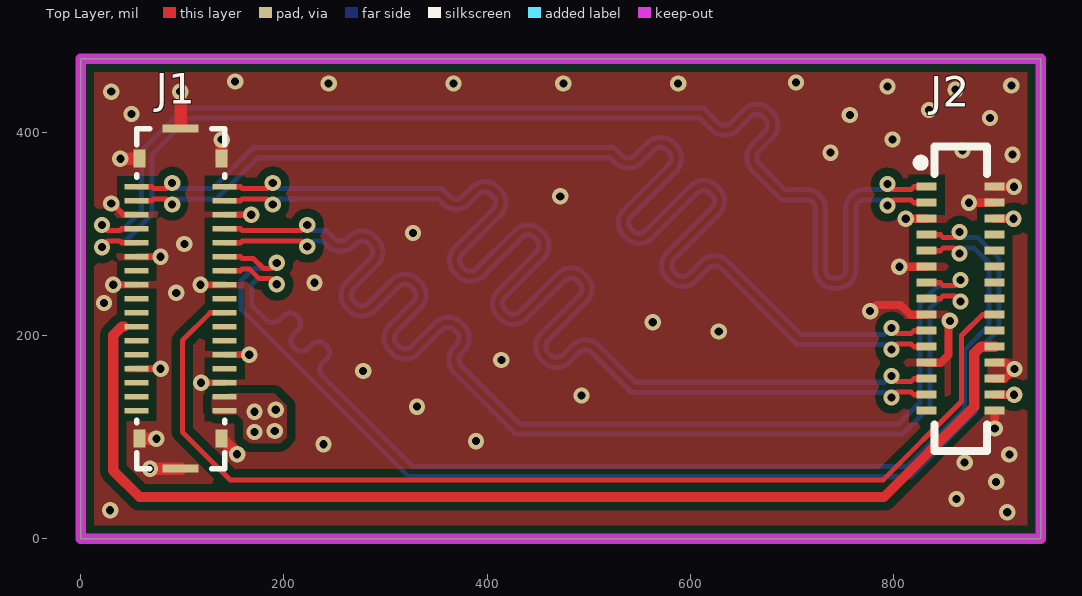
[diagram p0: Top Layer view]
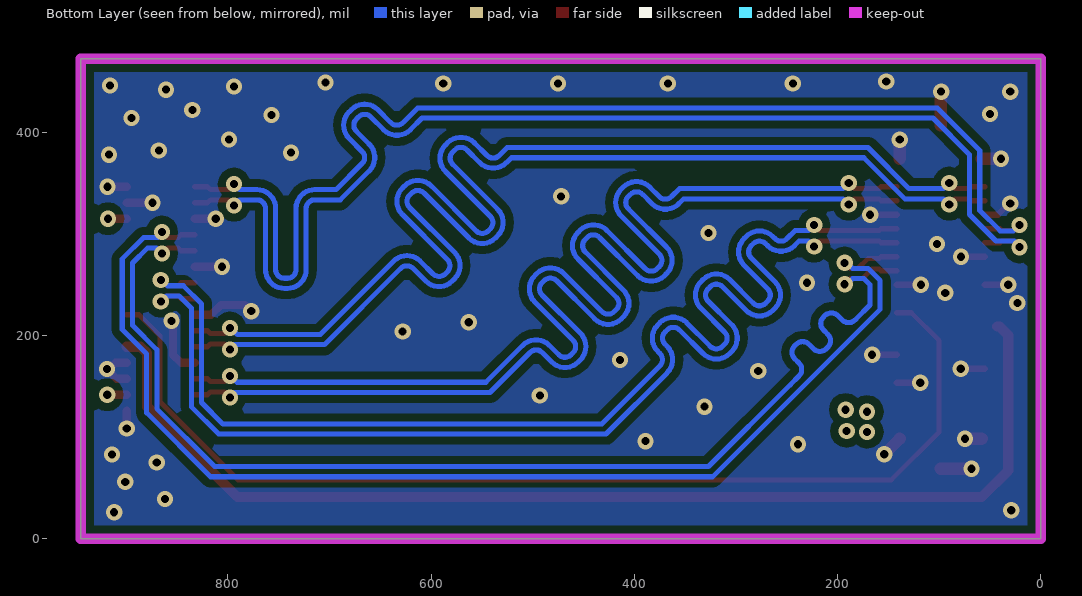
[diagram p1: Bottom Layer view, seen from below]
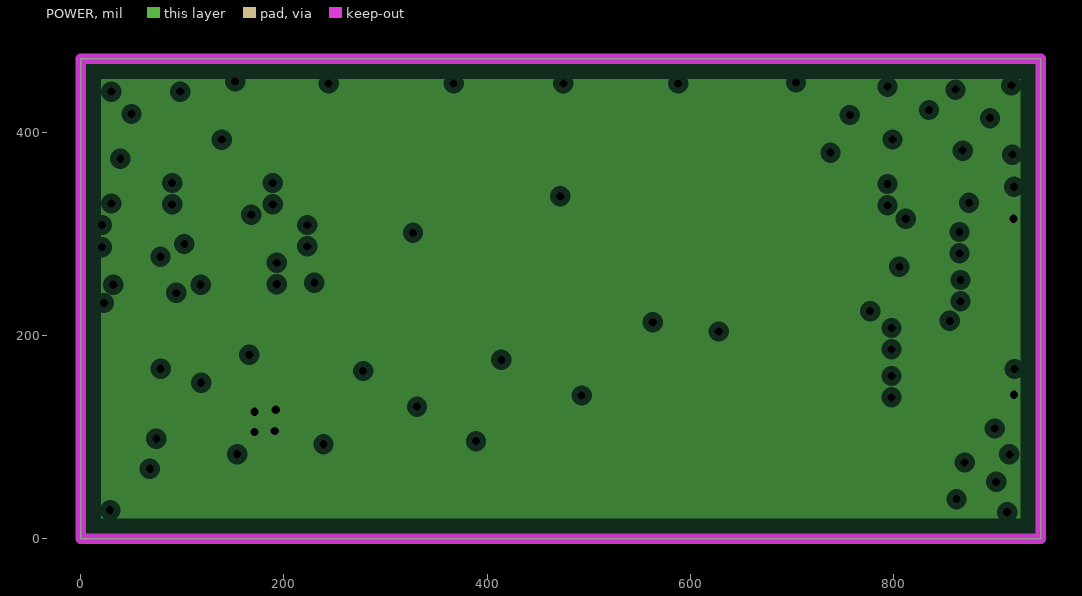
[diagram p2: POWER, clearances drawn from the general rule]
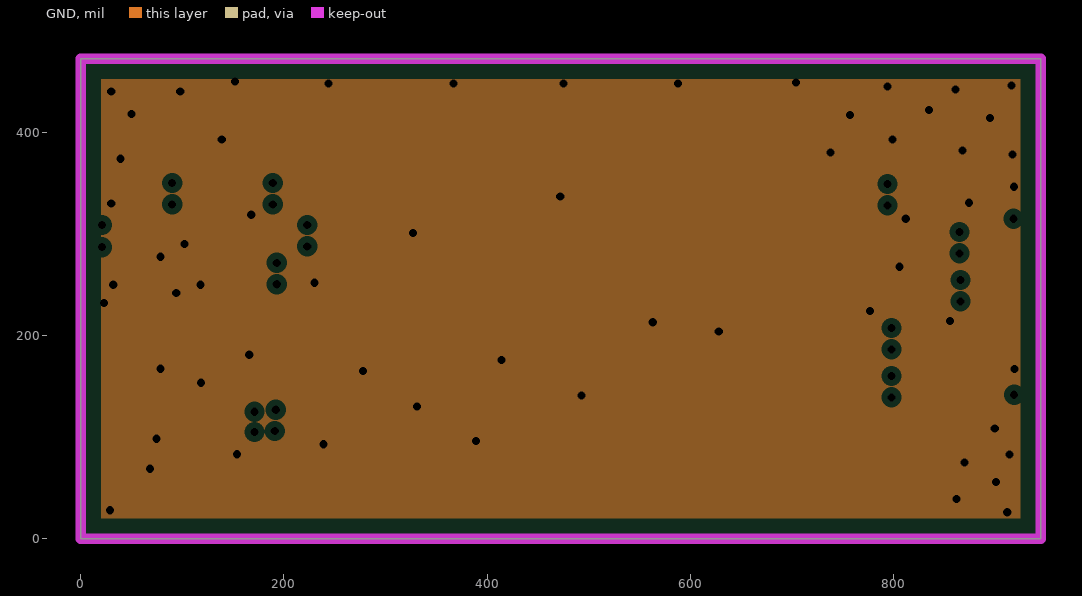
[diagram p3: GND, clearances drawn from the general rule]
# Altium PCB MISC89352-10.pcbdoc
Units mil, origin at the board's own origin, x right, y up, seen from the top; angles counter-clockwise.
Board outline 944.88 x 472.44 mil, 4 copper layers (Top Layer, POWER, GND, Bottom Layer); 2 components, 14 nets, 70 pads, 86 vias.

## Layer stack, top to bottom (the 12.6 mil dielectric is the usual default, probably not edited)
Top Layer: signal copper 1.4
Dielectric: core 12.6, FR-4, Dk 4.8
POWER: plane copper 1.4, net VDD_3V3
Dielectric: prepreg 12.6, FR-4, Dk 4.8
GND: plane copper 1.4, net GND
Dielectric: core 12.6, FR-4, Dk 4.8
Bottom Layer: signal copper 1.4

## Board outline
0,0 944.88,0 944.88,472.44 0,472.44

## Design rules (kind name [scope] priority, off if disabled: settings)
Clearance Clearance_1 [inpolygon] p1: gap=8
Clearance [All] p2: gap=5
DiffPairsRouting [All] p1: maxlimit=5 minlimit=5 mostfreqgap=5 maxuncoupledlength=500
HoleSize [All] p1: absolutevalues=TRUE maxlimit=500 minlimit=1 maxpercent=80.000 minpercent=20.000
HoleToHoleClearance [All] p1: gap=0 allowstackedmicrovias=TRUE
MinimumSolderMaskSliver [All] p1: minsoldermaskwidth=0
PlaneClearance [All] p1: clearance=6
PlaneConnect [All] p1: planeconnectstyle=Direct reliefexpansion=20 reliefentries=4 reliefconductorwidth=10 reliefairgap=10
PolygonConnect [All] p1: connectstyle=Direct reliefconductorwidth=10 reliefentries=4 polygonreliefangle="90 Angle"
RoutingVias [All] p1: holewidth=8 width=16 viastyle="Through Hole" minholewidth=8 minwidth=16 maxholewidth=8 maxwidth=16
SilkToSilkClearance [All] p1: silktosilkclearance=0
SilkscreenOverComponentPads [All] p1: minsilkscreentomaskgap=0
SolderMaskExpansion [All] p1: expansion=4
Width [All] p1: maxlimit=40 minlimit=5 preferedwidth=5 minimp=50.000000 maximp=50.000000 favimp=50.000000
20 further rules are at their usual default settings.

## Classes and differential pairs
differential pair D_MD0: +MDP0 -MDN0
differential pair D_MD1: +MDP1 -MDN1
differential pair D_CLK: +CLKP -CLKN
differential pair D_MD2: +MDP2 -MDN2
differential pair D_MD3: +MDP3 -MDN3

## Components (designator, comment, footprint, x,y, rotation, side; value= is the part's Value field where it differs from the comment)
J1 "BAF92-34073-0508" CONN-SMD_34P-P0.35_BAF92-34073-0508 98.43,236.22 r90 top locked
J2 "#NAME?" CONN-SMD_KYOCERA-AVX_145804030020829 866.14,236.22 r270 top locked

## Footprints (in the part's own frame and the unit in brackets; to place one, negate y for a bottom-side part, rotate by r counter-clockwise, add the part's x,y. Pads: shape width x height; smd on the part's side, far side on the other; paste and mask are expansions set on the pad)
CONN-SMD_34P-P0.35_BAF92-34073-0508 [mm]
  rect 0.13x0.6 smd paste+0 mask+0.05: 1(-2.8,1.1) 2(-2.45,1.1) 3(-2.1,1.1) 4(-1.75,1.1) 5(-1.4,1.1) 6(-1.05,1.1) 7(-0.7,1.1) 8(-0.35,1.1) 9(0,1.1) 10(0.35,1.1) 11(0.7,1.1) 12(1.05,1.1) 13(1.4,1.1) 14(1.75,1.1) 15(2.1,1.1) 16(2.45,1.1) 17(2.8,1.1) 18(2.8,-1.1) 19(2.45,-1.1) 20(2.1,-1.1) 21(1.75,-1.1) 22(1.4,-1.1) 23(1.05,-1.1) 24(0.7,-1.1) 25(0.35,-1.1) 26(0,-1.1) 27(-0.35,-1.1) 28(-0.7,-1.1) 29(-1.05,-1.1) 30(-1.4,-1.1) 31(-1.75,-1.1) 32(-2.1,-1.1) 33(-2.45,-1.1) 34(-2.8,-1.1)
  rect 0.45x0.3 smd paste+0 mask+0.05: 35(-3.5,1.025) 36(-3.5,-1.025) 37(3.5,-1.025) 38(3.5,1.025)
  rect 0.2x0.9 smd paste+0 mask+0.05: 39(-4.25,0) 40(4.25,0)
  silkscreen extent -4.25,-1.1 4.25,1.1
CONN-SMD_KYOCERA-AVX_145804030020829 [mm]
  rect 0.2x0.5 smd paste+0 mask+0.05: 1(-2.8,-0.85) 2(-2.8,0.85) 3(-2.4,-0.85) 4(-2.4,0.85) 5(-2,-0.85) 6(-2,0.85) 7(-1.6,-0.85) 8(-1.6,0.85) 9(-1.2,-0.85) 10(-1.2,0.85) 11(-0.8,-0.85) 12(-0.8,0.85) 13(-0.4,-0.85) 14(-0.4,0.85) 15(0,-0.85) 16(0,0.85) 17(0.4,-0.85) 18(0.4,0.85) 19(0.8,-0.85) 20(0.8,0.85) 21(1.2,-0.85) 22(1.2,0.85) 23(1.6,-0.85) 24(1.6,0.85) 25(2,-0.85) 26(2,0.85) 27(2.4,-0.85) 28(2.4,0.85) 29(2.8,-0.85) 30(2.8,0.85)
  silkscreen extent -3.8,-1.1 3.8,0.66

## Part data
J2: library part 14-5804-030-000-829

## Via types
v1: diameter 16, hole 8, Top Layer to Bottom Layer, 86 vias

## Nets (pads, with @x,y where several pads share a name; then routed paths per layer and width w, separated by ;. In a path a pad name is that pad's centre, name@x,y a point inside that pad or via, vN(x,y) a via of type N, cw(c..) or ccw(c..) an arc to the next point about the centre after c; other vN are vias at no path point)
AGND: J1.4 J1.10 J1.12 J1.15 J1.20 J1.25 J1.30 J1.32 J1.35 J1.36 J1.37 J1.38 J1.39 J1.40 J2.2 J2.4 J2.5 J2.11 J2.17 J2.23 J2.24 J2.26 J2.30 | length 609.8
  Top Layer w6: v1(30,330) 31,330 42.11,318.89 J1.15 ; v1(31.99,249.99) J1.10 ; J1.4 v1(78.69,167.31) ; J1.12 v1(78.55,277.55) ; v1(118.01,249.99) J1.25 ; v1(118.54,153.54) J1.32 ; J1.30 v1(165.9,181.1) ; J1.20 v1(167.89,318.89)
  Top Layer w8: v1(777,224) 783,230 807,230 816.52,220.48 J2.17 ; v1(805.72,267.72) J2.11 ; v1(812.03,314.97) J2.5 ; J2.23 846.23,173.23 854,181 854,213 v1(855.45,214.45) ; v1(874.29,330.71) J2.4 ; v1(899.6,108.4) J2.30 ; J2.26 909.49,157.49 v1(919,167) ; J2.24 910.77,173.23 v1@917,167 ; J2.2 v1(918.54,346.46)
  Top Layer w12: v1(39.01,374.01) J1.38 ; J1.35 v1(74.42,98.42) ; v1(68.1,68.9) J1.39 ; v1(98,440) 98.43,439.57 J1.40@98.43,407 ; J1.36 v1(154,83.19) ; J1.37 v1(138.77,392.77)
  other v1: 912,26 29,28 862,39 901,56 870,75 914,83 239,93 389,96 331,130 493,141 278,165 414,176 628,204 563,213 23,232 94,242 230,252 102,290 327,301 472,337 917,378 738,380 868,382 799,393 895,414 757,417 50,418 835,422 30,440 861,442 794,445 916,446 244,448 367,448 475,448 588,448 704,449 152,450
CLKN: J1.19 J2.27 | length 1181.7
  Top Layer w5: J1.19 157,332.67 158.89,334.56 183.5,334.56 v1(189,329.06) ; v1(798,139.11) 803.5,144.61 817.12,144.61 820,141.74 J2.27
  Bottom Layer w5: v1(189,329.06) 194.5,334.56 351.44,334.56 356.34,329.66 ccw(c369.42,342.74) 382.5,329.66 391.82,338.98 cw(c397.83,332.97) 403.84,338.98 405.96,336.86 cw(c399.95,330.85) 408.45,330.85 cw(c399.95,330.85) 405.96,324.84 368.23,287.11 ccw(c381.31,274.03) 368.23,260.94 370.35,258.82 ccw(c383.44,271.91) 396.52,258.82 434.25,296.55 cw(c440.26,290.54) 446.27,296.55 448.39,294.43 cw(c442.38,288.42) 450.88,288.42 cw(c442.38,288.42) 448.39,282.41 410.66,244.68 ccw(c423.74,231.6) 410.66,218.52 412.78,216.4 ccw(c425.86,229.48) 438.94,216.4 476.67,254.13 cw(c482.68,248.12) 488.69,254.13 490.82,252.01 cw(c484.81,246) 493.31,246 cw(c484.81,246) 490.83,239.99 ; 490.82,239.99 453.09,202.26 ccw(c466.17,189.17) 453.09,176.09 455.21,173.97 ccw(c468.29,187.05) 481.37,173.97 490.69,183.29 cw(c496.7,177.28) 502.71,183.29 542,144 793.11,144 v1(798,139.11)
CLKP: J1.18 J2.25 | length 1182.3
  Top Layer w5: J1.18 157,346.45 158.89,344.56 183.5,344.56 v1(189,350.06) ; v1(798,160.11) 803.5,154.61 817.12,154.61 820,157.49 J2.25
  Bottom Layer w5: v1(189,350.06) 194.5,344.56 355.58,344.56 363.41,336.73 ccw(c369.42,342.74) 375.43,336.73 384.75,346.05 cw(c397.83,332.97) 410.91,346.05 413.03,343.93 cw(c399.95,330.85) 418.45,330.85 cw(c399.95,330.85) 413.03,317.77 375.29,280.03 ccw(c381.31,274.03) 375.3,268.02 377.43,265.89 ccw(c383.44,271.91) 389.45,265.89 427.18,303.62 cw(c440.26,290.54) 453.34,303.62 455.46,301.5 cw(c442.38,288.42) 460.88,288.42 cw(c442.38,288.42) 455.46,275.34 417.72,237.6 ccw(c423.74,231.6) 417.73,225.59 419.86,223.46 ccw(c425.86,229.48) 431.87,223.47 469.6,261.2 cw(c482.68,248.12) 495.77,261.2 497.89,259.08 cw(c484.81,246) 503.31,246 cw(c484.81,246) 497.89,232.91 460.15,195.17 ccw(c466.17,189.17) 460.16,183.16 462.28,181.04 ccw(c468.29,187.05) 474.3,181.04 483.62,190.36 cw(c496.7,177.28) 509.78,190.36 546.14,154 790.97,154 797.08,160.11 v1(798,160.11)
MDN0: J1.24 J2.9 | length 1182
  Top Layer w5: J1.24 157,263.77 158.89,265.66 166,265.66 175.66,256 v1@187.5,256 ; J2.9 846,283.47 848.88,286.34 859.5,286.34 v1(865,280.84)
  Bottom Layer w5: v1@191,250 185,256 174,256 168,250 168,230 182,216 182.71,215.29 ccw(c189.07,221.66) 195.44,215.29 199.74,219.6 cw(c206.1,213.23) 212.47,219.6 213.88,218.18 cw(c207.52,211.82) 213.88,205.46 209.58,201.15 ccw(c215.94,194.79) 209.58,188.42 210.99,187.01 ccw(c217.36,193.37) 223.72,187.01 228.02,191.31 cw(c234.39,184.95) 240.75,191.31 242.17,189.9 cw(c235.8,183.53) 242.17,177.17 237.86,172.87 ccw(c244.23,166.5) 237.86,160.14 246.5,151.5 327,71 813,71 870,128 870,186 894,210 894,271.34 879,286.34 870.5,286.34 v1(865,280.84)
  other v1: 193,250.5
MDN1: J1.22 J2.15 | length 1184.3
  Top Layer w5: J1.22 157,291.33 158.89,293.22 217.5,293.22 v1(223,287.72) ; J2.15 846,236.22 848.88,239.09 v1@860.5,239.09
  Bottom Layer w5: v1(223,287.72) 228.5,293.22 237.64,293.22 242.54,288.32 ccw(c255.62,301.4) 268.7,288.32 270.83,290.45 cw(c276.83,284.43) 282.84,290.44 284.96,288.32 cw(c278.95,282.31) 287.45,282.31 cw(c278.95,282.31) 284.97,276.31 261.63,252.97 ccw(c274.71,239.88) 261.63,226.8 263.75,224.68 ccw(c276.83,237.76) 289.91,224.68 313.25,248.02 cw(c319.26,242.01) 325.27,248.02 327.39,245.89 cw(c321.38,239.88) 329.88,239.88 cw(c321.38,239.88) 327.4,233.88 304.06,210.54 ccw(c317.14,197.46) 304.06,184.38 306.18,182.25 ccw(c319.26,195.34) 332.34,182.25 355.67,205.59 cw(c361.68,199.58) 367.69,205.59 369.82,203.47 cw(c363.81,197.46) 372.31,197.46 cw(c363.81,197.46) 369.83,191.46 367.69,189.33 ccw(c380.78,176.24) 367.69,163.16 427.86,103 809.14,103 836,129.86 836,227 848,239 855,239 ; 856,239 855,239 ; v1(866,233.59) 860.59,239 855,239
MDN2: J1.13 J2.3 | length 1182.2
  Top Layer w5: 26.5,293.22 38.11,293.22 40,291.33 J1.13 ; v1(794,328.08) 799.5,333.58 817.12,333.58 820,330.71 J2.3
  Bottom Layer w5: v1@23,290 26,293 44,293 70,319 70,378 106,414 609,414 620.56,402.44 ccw(c633.64,415.52) 646.72,402.44 659.45,415.17 ; 659.47,415.18 cw(c665.46,409.16) 671.47,415.17 673.59,413.05 cw(c667.58,407.04) 676.08,407.04 cw(c667.58,407.04) 673.59,401.03 ; 673.59,401.03 660.87,388.3 ccw(c673.95,375.22) 660.87,362.13 689.42,333.58 714.5,333.58 cw(c714.5,325.08) 723,325.08 723,264.84 ccw(c741.5,264.84) 741.5,246.34 744.5,246.34 ccw(c744.5,264.84) 763,264.84 763,325.08 cw(c771.5,325.08) 771.5,333.58 788.5,333.58 v1(794,328.08)
  other v1: 21,287
MDN3: J1.16 J2.21 | length 1181.6
  Top Layer w5: J1.16 70,332.67 71.89,334.56 84.5,334.56 v1(90,329.06) ; v1(798,186.35) 803.5,191.85 817.12,191.85 820,188.98 J2.21
  Bottom Layer w5: v1(90,329.06) 95.5,334.56 133.7,334.56 174.14,375 521,375 525.9,370.1 ccw(c538.98,383.18) 552.06,370.1 564.64,382.68 cw(c570.65,376.67) 576.66,382.68 578.78,380.56 cw(c572.77,374.55) 581.27,374.55 cw(c572.77,374.55) 578.78,368.54 534.53,324.29 ccw(c547.61,311.21) 534.53,298.12 536.65,296 ccw(c549.74,309.08) 562.82,296 607.07,340.25 cw(c613.08,334.24) 619.09,340.25 621.21,338.13 cw(c615.2,332.12) 623.7,332.12 cw(c615.2,332.12) 621.21,326.11 576.96,281.86 ccw(c590.04,268.78) 576.96,255.7 579.08,253.58 ccw(c592.16,266.66) 605.24,253.58 617.83,266.17 cw(c623.83,260.15) 629.84,266.16 705,191 793.35,191 v1(798,186.35)
MDP0: J1.23 J2.7 | length 1182.3
  Top Layer w5: J1.23 157,277.55 158.89,275.66 170.14,275.66 179.8,266 v1@187.5,266 ; J2.7 846,299.22 848.88,296.34 859.5,296.34 v1(865,301.84)
  Bottom Layer w5: v1@190,271 185,266 169.86,266 158,254.14 158,225.86 322.86,61 817.14,61 880,123.86 880,181.86 904,205.86 904,275.48 883.14,296.34 869,296.34 865,300.34 v1(865,301.84)
  other v1: 193,271.5
MDP1: J1.21 J2.13 | length 1184.4
  Top Layer w5: J1.21 157,305.11 158.89,303.22 217.5,303.22 v1(223,308.72) ; J2.13 846,251.97 848.88,249.09 v1@860.5,249.09
  Bottom Layer w5: v1(223,308.72) 228.5,303.22 241.78,303.22 249.61,295.39 ccw(c255.62,301.4) 261.63,295.39 263.75,297.51 cw(c276.83,284.43) 289.91,297.51 292.03,295.39 cw(c278.95,282.31) 297.45,282.31 cw(c278.95,282.31) 292.03,269.23 268.7,245.89 ccw(c274.71,239.88) 268.7,233.87 270.82,231.75 ccw(c276.83,237.76) 282.82,231.73 ; 282.83,231.74 306.18,255.09 cw(c319.26,242.01) 332.34,255.09 334.46,252.97 cw(c321.38,239.88) 339.88,239.88 cw(c321.38,239.88) 334.46,226.8 311.13,203.47 ccw(c317.14,197.46) 311.13,191.45 313.25,189.33 ccw(c319.26,195.34) 325.25,189.31 348.6,212.66 cw(c361.68,199.58) 374.77,212.66 376.89,210.54 cw(c363.81,197.46) 382.31,197.46 cw(c363.81,197.46) 376.89,184.38 374.77,182.25 ccw(c380.78,176.24) 374.77,170.23 432,113 805,113 826,134 826,231.14 843.86,249 855,249 ; 856,249 855,249 ; v1(866,254.59) 865.08,254.59 859.49,249 855,249
MDP2: J1.14 J2.1 | length 1181.8
  Top Layer w5: v1@26.5,303.22 38.11,303.22 40,305.11 J1.14 ; v1(794,349.08) 799.5,343.58 817.12,343.58 820,346.46 J2.1
  Bottom Layer w5: v1@24,306 26.78,303.22 27.42,303.22 27.64,303 ; 27,303 39.86,303 60,323.14 60,382.14 101.86,424 613.14,424 627.63,409.51 ccw(c633.64,415.52) 639.65,409.51 652.38,422.24 cw(c665.46,409.16) 678.54,422.24 680.66,420.12 cw(c667.58,407.04) 686.08,407.04 cw(c667.58,407.04) 680.66,393.95 667.93,381.22 ccw(c673.95,375.22) 667.94,369.21 693.56,343.58 714.5,343.58 cw(c714.5,325.08) 733,325.08 733,264.84 ccw(c741.5,264.84) 741.5,256.34 744.5,256.34 ccw(c744.5,264.84) 753,264.84 753,325.08 cw(c771.5,325.08) 771.5,343.58 788.5,343.58 v1(794,349.08)
  other v1: 21,308.72
MDP3: J1.17 J2.19 | length 1182.4
  Top Layer w5: J1.17 70,346.45 71.89,344.56 84.5,344.56 v1(90,350.06) ; v1(798,207.35) 803.5,201.85 817.12,201.85 820,204.73 J2.19
  Bottom Layer w5: v1(90,350.06) 95.5,344.56 129.56,344.56 170,385 525.14,385 532.97,377.17 ccw(c538.98,383.18) 544.99,377.17 557.57,389.75 cw(c570.65,376.67) 583.73,389.75 585.86,387.63 cw(c572.77,374.55) 591.27,374.55 cw(c572.77,374.55) 585.86,361.47 541.6,317.22 ccw(c547.61,311.21) 541.6,305.19 543.73,303.07 ccw(c549.74,309.08) 555.75,303.07 600,347.33 cw(c613.08,334.24) 626.16,347.33 628.28,345.2 cw(c615.2,332.12) 633.7,332.12 cw(c615.2,332.12) 628.28,319.04 584.03,274.79 ccw(c590.04,268.78) 584.03,262.77 586.16,260.64 ccw(c592.16,266.66) 598.17,260.65 610.75,273.23 cw(c623.83,260.15) 636.92,273.23 709.14,201 790.73,201 797.08,207.35 v1(798,207.35)
RESET: J1.27 J2.18 | length 1067.5
  Top Layer w5: J1.27 127.44,222.44 100,195 100,105 147,58 790,58 867,135 867,200 887.48,220.48 J2.18
VDD_1V8: J1.7 J2.22 | length 1118.4
  Top Layer w10: 43,209 40.74,209 32,200.26 32,67 58,41 790.68,41 879.5,129.82 879.5,182.5 885.98,188.98 J2.22
VDD_3V3: J1.33 J1.34 J2.6 J2.28 | length 37.6
  Top Layer w8: J2.28 v1(918.74,141.74) ; J2.6 v1(918.03,314.97)
  other v1: 171,105 191,106 171,125 192,127
pads on no net: J1.1 J1.2 J1.3 J1.5 J1.6 J1.8 J1.9 J1.11 J1.26 J1.28 J1.29 J1.31 J2.8 J2.10 J2.12 J2.14 J2.16 J2.20 J2.29

## Polygon pours and split planes (outlines as drawn)
AGND on Top Layer "Bottom Layer-No Net" (solid, remove dead copper): -62,426 -62,-29 -31,-60 -26,-65 1,-65 981,-65 989,-57 1033,-13 1033,96 1033,487 992,528 974,546 952,546 0,546 -29,517 -62,484 -62,427
VDD_3V3 on Top Layer "Bottom Layer-No Net" (solid, remove dead copper): 129,137 129,125 131,123 132,122 141,122 154,122 158,118 160,116 160,106 160,99 163,96 165,94 169,94 197,94 200,97 203,100 203,102 203,131 197,137 191,143 158,143 132,143 130,141 129,140 129,137
AGND on Bottom Layer "Bottom Layer-No Net" (solid, remove dead copper): -83,449 -83,-34 -25,-92 5,-122 120,-122 986,-122 1062,-46 1085,-23 1085,-5 1085,493 1016,562 981,597 968,597 -9,597 -46,560 -81,525 -81,463
VDD_3V3 on POWER (split plane): 924.79,20.1 20.1,20.1 20.1,452.34 924.79,452.34
AGND on GND (split plane): 924.79,20.1 20.1,20.1 20.1,452.34 924.79,452.34

## Keep-outs
Board Outline Layer:
  the board outline again, w10